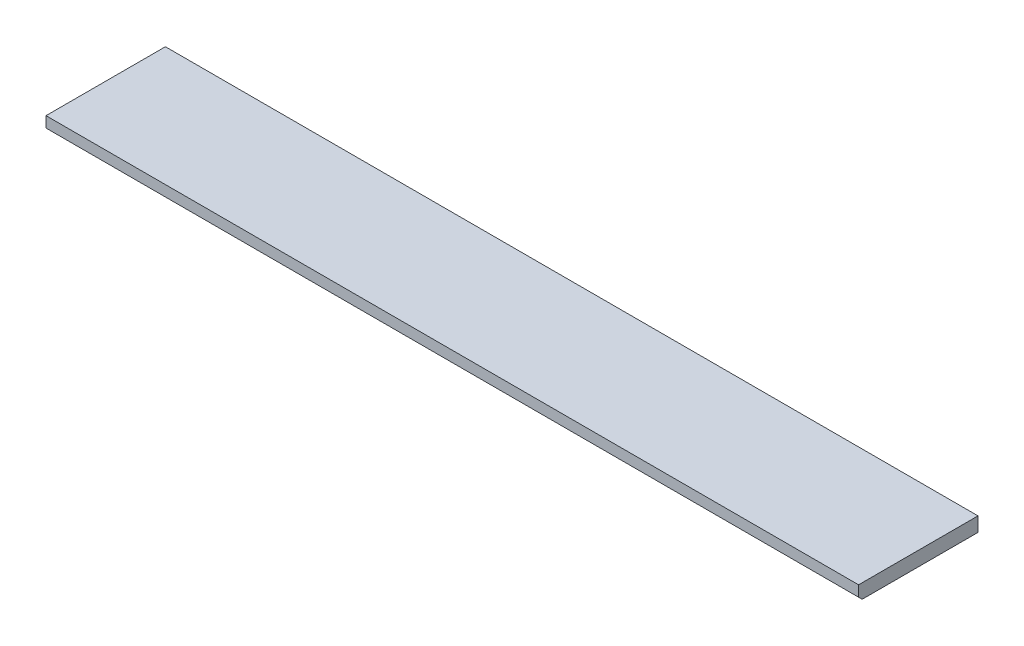
from build123d import *

# Parameters (mm, degrees)
SKETCH_1_W      = 2266
SKETCH_1_H      = 333
EXTRUDE_1_DEPTH = 40
CHAMFER_1_SIZE  = 10


with BuildPart() as part:
    # 草图1 → 凸台-拉伸1 (new body)
    with BuildSketch(Plane(origin=(0, 0, 0), x_dir=(1, 0, 0), z_dir=(0, 1, 0))):
        Rectangle(SKETCH_1_W, SKETCH_1_H)
    extrude(amount=EXTRUDE_1_DEPTH)

    # 倒角1
    chamfer_1_edges = [part.edges().sort_by_distance(p)[0] for p in [
        (0, 0, 166.5),
    ]]
    chamfer(chamfer_1_edges, length=CHAMFER_1_SIZE)


solid = part.part
